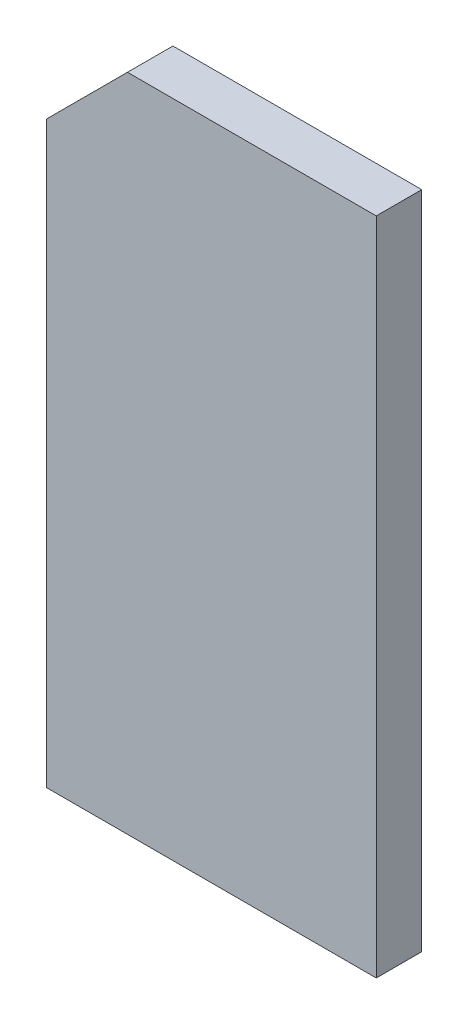
from build123d import *

# Parameters (mm, degrees)
SKETCH1_W      = 101.6
SKETCH1_H      = 203.2
EXTRUDE1_DEPTH = 7
CHAMFER1_SIZE  = 25


with BuildPart() as part:
    # Sketch1 → Extrude1 (new, symmetric)
    with BuildSketch(Plane.XY):
        with Locations((50.8, 101.6)):
            Rectangle(SKETCH1_W, SKETCH1_H)
    extrude(amount=EXTRUDE1_DEPTH, both=True)

    # Chamfer1
    chamfer1_edges = [part.edges().sort_by_distance(p)[0] for p in [
        (0, 203.2, 0),
    ]]
    chamfer(chamfer1_edges, length=CHAMFER1_SIZE)


solid = part.part
